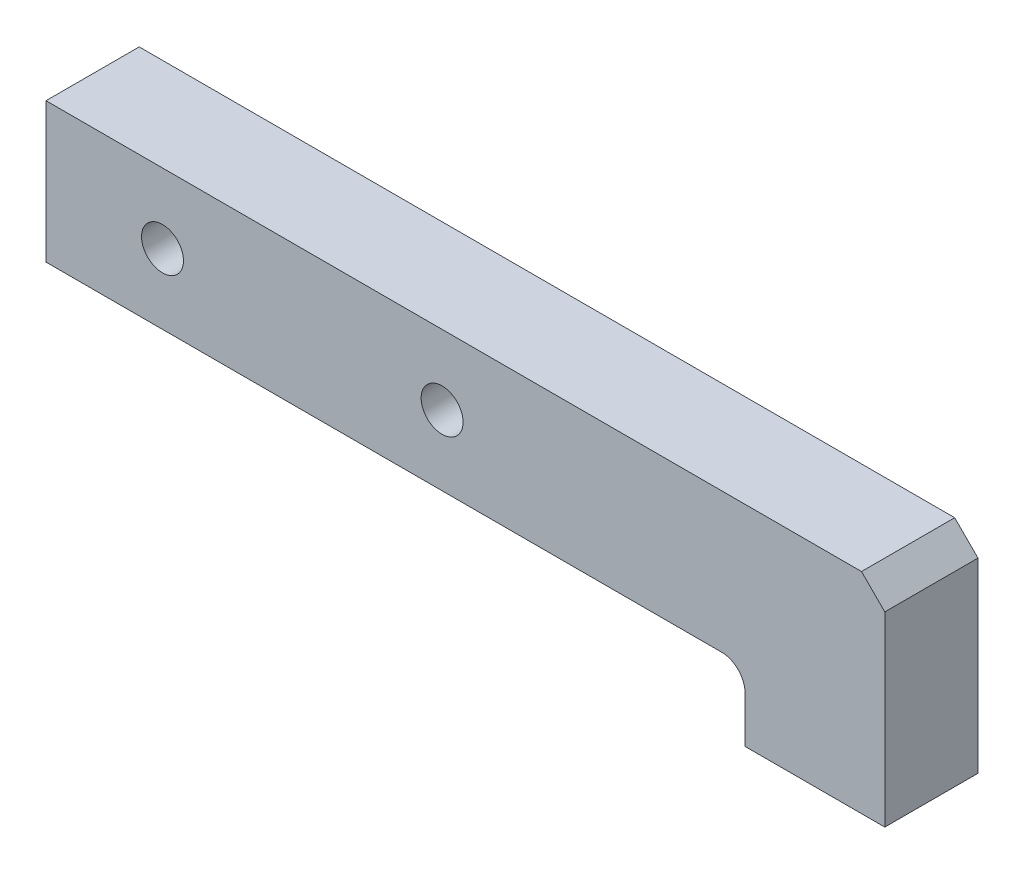
from build123d import *

# Parameters (mm, degrees)
SKETCH_1_W                = 180
SKETCH_1_H                = 30
EXTRUDE_1_DEPTH           = 20
SKETCH_4_W                = 30
SKETCH_4_H                = 15
EXTRUDE_2_DEPTH           = 20
FILLET_1_R                = 5
CHAMFER_1_SIZE            = 5
HOLE_WIZARD_M8_2_D        = 6.8
HOLE_WIZARD_M8_2_DEPTH    = 19.75
HOLE_WIZARD_M8_2_TIP      = 2.042926105
HOLE_WIZARD_1_D           = 9
HOLE_WIZARD_1_DEPTH       = 27.5
HOLE_WIZARD_1_CBORE_D     = 15
HOLE_WIZARD_1_CBORE_DEPTH = 9
HOLE_WIZARD_1_TIP         = 2.703872786


with BuildPart() as part:
    # 草图1 → 凸台-拉伸1 (new body)
    with BuildSketch(Plane.XY):
        Rectangle(SKETCH_1_W, SKETCH_1_H)
    extrude(amount=EXTRUDE_1_DEPTH)

    # 草图4 → 凸台-拉伸2 (add)
    with BuildSketch(Plane.XY.offset(20)):
        with Locations((75, -22.5)):
            Rectangle(SKETCH_4_W, SKETCH_4_H)
    extrude(amount=-EXTRUDE_2_DEPTH)

    # 圆角1
    fillet_1_edges = [part.edges().sort_by_distance(p)[0] for p in [
        (60, -15, 10),
    ]]
    fillet(fillet_1_edges, radius=FILLET_1_R)

    # 倒角1
    chamfer_1_edges = [part.edges().sort_by_distance(p)[0] for p in [
        (90, 15, 10),
    ]]
    chamfer(chamfer_1_edges, length=CHAMFER_1_SIZE)

    # M8 螺纹孔2
    with Locations(Plane(origin=(0, -30, 0), x_dir=(-1, 0, 0), z_dir=(0, -1, 0))):
        with Locations((-75, -10)):
            Hole(HOLE_WIZARD_M8_2_D / 2, depth=HOLE_WIZARD_M8_2_DEPTH)
            with Locations((0, 0, -(HOLE_WIZARD_M8_2_DEPTH + HOLE_WIZARD_M8_2_TIP / 2))):  # 118° drill point
                Cone(0, HOLE_WIZARD_M8_2_D / 2, HOLE_WIZARD_M8_2_TIP, mode=Mode.SUBTRACT)

    # 打孔尺寸(%根据)内六角圆柱头螺钉的类型1
    with Locations(Plane(origin=(0, 0, 0), x_dir=(-1, 0, 0), z_dir=(0, 0, -1))):
        with Locations((65, 0), (5, 0)):
            CounterBoreHole(HOLE_WIZARD_1_D / 2, HOLE_WIZARD_1_CBORE_D / 2, HOLE_WIZARD_1_CBORE_DEPTH, depth=HOLE_WIZARD_1_DEPTH)
            with Locations((0, 0, -(HOLE_WIZARD_1_DEPTH + HOLE_WIZARD_1_TIP / 2))):  # 118° drill point
                Cone(0, HOLE_WIZARD_1_D / 2, HOLE_WIZARD_1_TIP, mode=Mode.SUBTRACT)


solid = part.part
